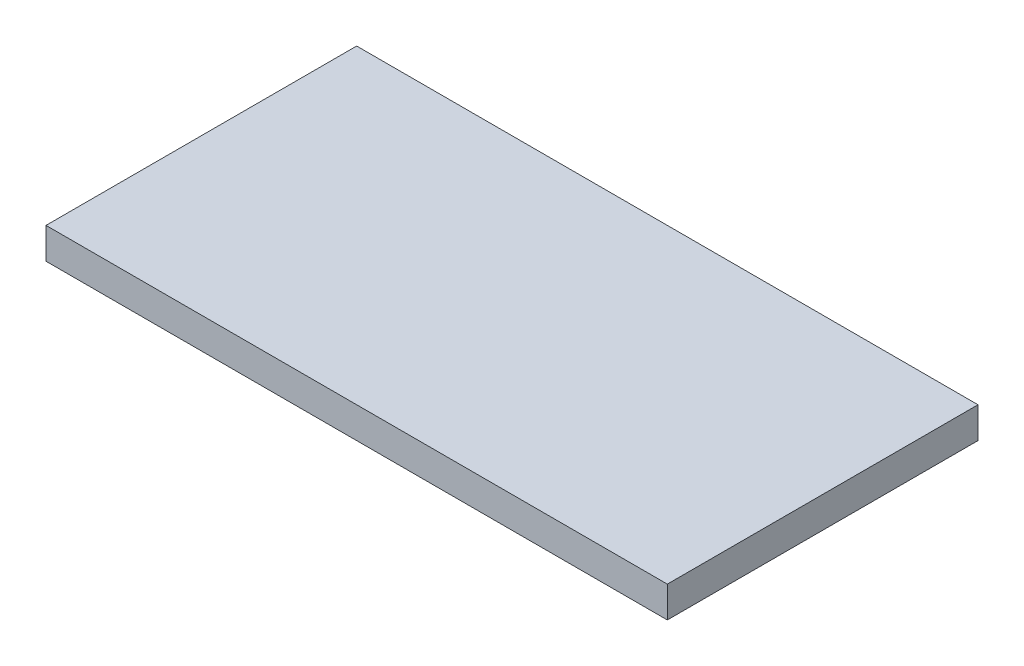
SolidWorks part; units mm, degrees
ref_plane "前视基准面" through (0, 0, 0) normal (0, 0, 1) x (1, 0, 0)
ref_plane "上视基准面" through (0, 0, 0) normal (0, 1, 0) x (1, 0, 0)
ref_plane "右视基准面" through (0, 0, 0) normal (1, 0, 0) x (0, 0, -1)
sketch "草图1" plane through (0, 0, 0) normal (0, 1, 0) x (1, 0, 0)
  line L1 (-500, 250) -> (500, 250)
  line L2 (-500, 250) -> (-500, -250)
  line L3 (-500, -250) -> (500, -250)
  line L4 (500, 250) -> (500, -250)
  line L5 (-500, 250) -> (500, -250) construction
  line L6 (-500, -250) -> (500, 250) construction
  point P0 (0, 0)
  dimension "D1" = 1000
  dimension "D2" = 500
extrude "凸台-拉伸1" add sketch "草图1" along normal blind 50
